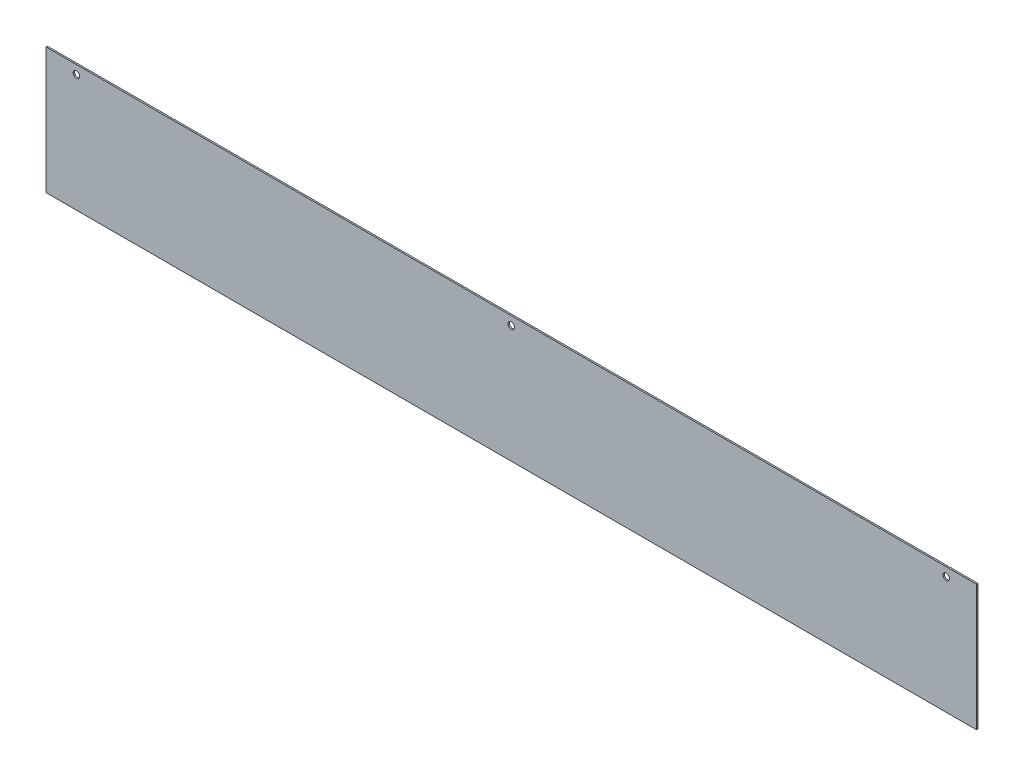
from build123d import *

# Parameters (mm, degrees)
SKETCH1_W          = 642
SKETCH1_H          = 1
EXTRUDE1_DEPTH     = 43.5
SKETCH2_R          = 2.25
CUT_EXTRUDE1_DEPTH = 324.93556458


with BuildPart() as part:
    # Sketch1 → Extrude1 (new, symmetric)
    with BuildSketch(Plane(origin=(0, 0, 0), x_dir=(1, 0, 0), z_dir=(0, 1, 0))):
        Rectangle(SKETCH1_W, SKETCH1_H)
    extrude(amount=EXTRUDE1_DEPTH, both=True)

    # Sketch2 → Cut-Extrude1 (cut, through all)
    with BuildSketch(Plane.XY.offset(0.5)):
        with Locations((-300, 37.5)):
            Circle(SKETCH2_R)
        with Locations((0, 37.5)):
            Circle(SKETCH2_R)
        with Locations(Location((300, 37.5, 0), (0, 0, 180))):
            Circle(SKETCH2_R)
    extrude(amount=-CUT_EXTRUDE1_DEPTH, mode=Mode.SUBTRACT)


solid = part.part
